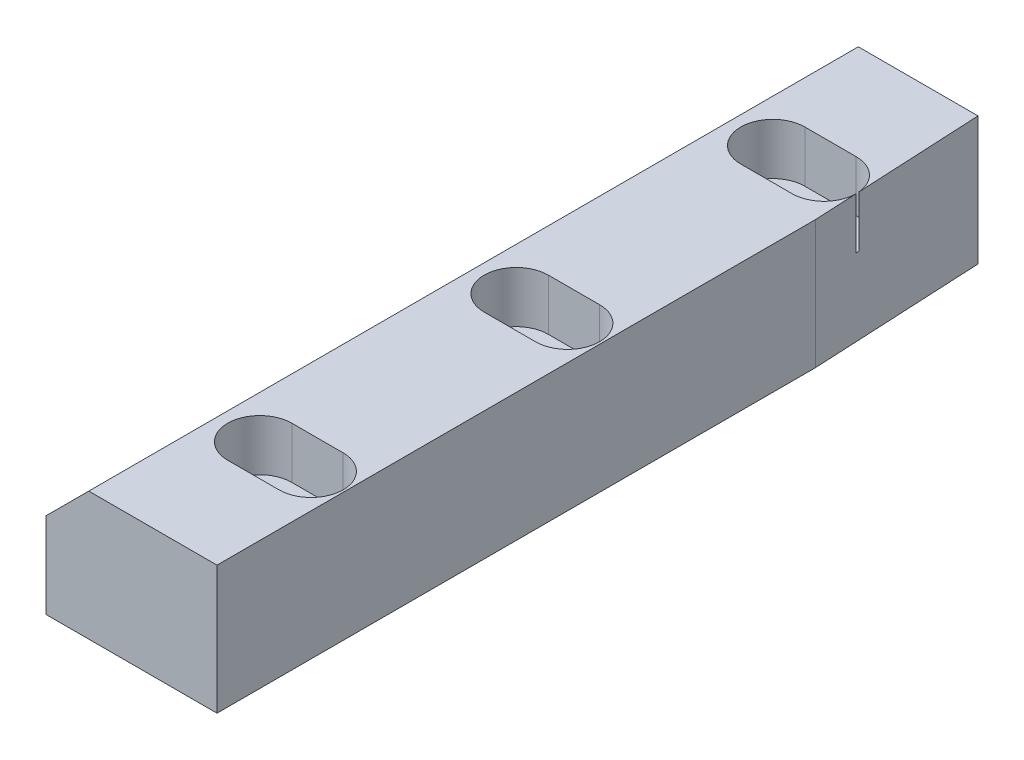
SolidWorks part; units mm, degrees
ref_plane "Front Plane" through (0, 0, 0) normal (0, 0, 1) x (1, 0, 0)
ref_plane "Top Plane" through (0, 0, 0) normal (0, 1, 0) x (1, 0, 0)
ref_plane "Right Plane" through (0, 0, 0) normal (1, 0, 0) x (0, 0, -1)
sketch "Sketch1" plane through (0, 0, 0) normal (0, 1, 0) x (1, 0, 0)
  line L1 (-10, 45) -> (10, 45)
  line L2 (-10, 45) -> (-10, -45)
  line L3 (-10, -45) -> (10, -45)
  line L4 (10, 45) -> (10, -45)
  line L5 (-10, 45) -> (10, -45) construction
  line L6 (-10, -45) -> (10, 45) construction
  point P0 (0, 0)
  dimension "D1" = 20
  dimension "D2" = 90
extrude "Boss-Extrude1" add sketch "Sketch1" along normal blind 15
chamfer "Chamfer1" distance 5 angle 45 1 edges at (-10, 15, 0)
sketch "Sketch2" plane through (0, 15, 0) normal (0, 1, 0) x (1, 0, 0)
  line L0 (10, 25) -> (9, 45)
  line L1 (10, -45) -> (10, 45) construction
  line L2 (10, 45) -> (-5, 45) construction
  line L3 (9, 45) -> (10, 45)
  line L4 (10, 45) -> (10, 25)
  dimension "D1" = 1
  dimension "D2" = 20
extrude "Cut-Extrude1" cut sketch "Sketch2" against normal through all
sketch "Sketch3" plane through (0, 15, 0) normal (0, 1, 0) x (1, 0, 0)
  line L0 (0, 0) -> (6, 0) construction
  line L1 (0, 2.25) -> (6, 2.25)
  line L2 (0, -2.25) -> (6, -2.25)
  arc A0 (0, 2.25) -> (0, -2.25) centre (0, 0) ccw
  arc A1 (6, -2.25) -> (6, 2.25) centre (6, 0) ccw
  point P3 (3, 0)
  dimension "D1" = 6
  dimension "D2" = 4.5
extrude "Cut-Extrude2" cut sketch "Sketch3" against normal through all
sketch "Sketch4" plane through (0, 15, 0) normal (0, 1, 0) x (1, 0, 0)
  line L4 (0, -3.75) -> (6, -3.75)
  line L5 (6, 3.75) -> (0, 3.75)
  line L6 (0, -3.75) -> (6, -3.75)
  line L7 (6, 3.75) -> (0, 3.75)
  arc A4 (0, 3.75) -> (0, -3.75) centre (0, 0) ccw
  arc A5 (6, -3.75) -> (6, 3.75) centre (6, 0) ccw
  arc A6 (0, 3.75) -> (0, -3.75) centre (0, 0) ccw
  arc A7 (6, -3.75) -> (6, 3.75) centre (6, 0) ccw
  dimension "D1" = 1.5
extrude "Cut-Extrude3" cut sketch "Sketch4" against normal blind 6
pattern_linear "Linear pattern1" count 2 spacing 30 along (0, 0, 1) count 2 spacing 30 along (0, 0, -1) seed only of "Cut-Extrude3", "Cut-Extrude2"
